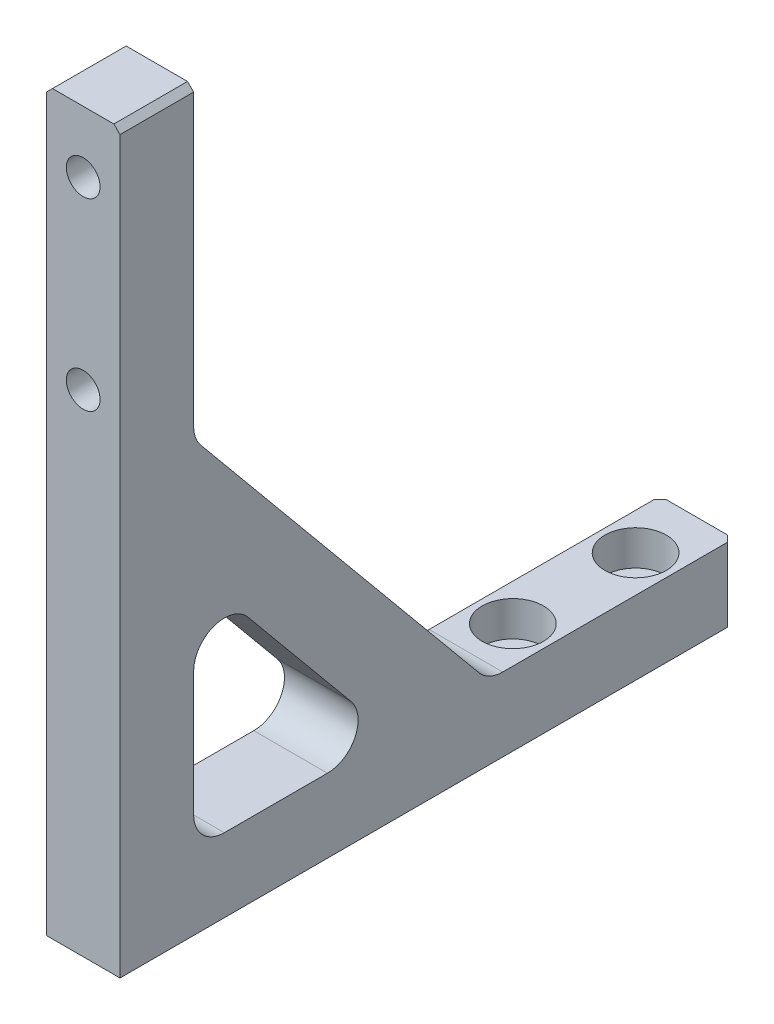
SolidWorks part; units mm, degrees
material "AL6061"
ref_plane "Front Plane" through (0, 0, 0) normal (0, 0, 1) x (1, 0, 0)
ref_plane "Top Plane" through (0, 0, 0) normal (0, 1, 0) x (1, 0, 0)
ref_plane "Right Plane" through (0, 0, 0) normal (1, 0, 0) x (0, 0, -1)
sketch "Sketch1" plane through (0, 0, 0) normal (1, 0, 0) x (0, 0, -1)
  line L0 (0, 0) -> (0, 120)
  line L1 (0, 120) -> (12, 120)
  line L2 (12, 120) -> (12, 70)
  line L3 (12, 70) -> (60, 12)
  line L4 (60, 12) -> (100, 12)
  line L5 (100, 12) -> (100, 0)
  line L6 (100, 0) -> (0, 0)
  dimension "D1" = 12
  dimension "D2" = 12
  dimension "D3" = 120
  dimension "D4" = 100
  dimension "D5" = 40
  dimension "D6" = 50
extrude "Boss-Extrude1" add sketch "Sketch1" along normal blind 12
sketch "Sketch2" plane through (12, 0, 0) normal (1, 0, 0) x (0, 0, -1)
  line L0 (12, 37.2945) -> (12, 17)
  line L1 (17, 12) -> (33.7954, 12)
  line L2 (37.6474, 20.1878) -> (20.852, 40.4823)
  line L3 (12, 70) -> (12, 120) construction
  line L4 (100, 12) -> (60, 12) construction
  line L6 (60, 12) -> (12, 70) construction
  arc A0 (33.7954, 12) -> (37.6474, 20.1878) centre (33.7954, 17) ccw
  arc A1 (12, 17) -> (17, 12) centre (17, 17) ccw
  arc A2 (12, 37.2945) -> (20.852, 40.4823) centre (17, 37.2945) cw
  dimension "D2" = 5
  dimension "D1" = 12
extrude "Cut-Extrude1" cut sketch "Sketch2" against normal through all
hole_wizard "CBORE for M5 Hexagon socket head cap screws1" positions "Sketch3" profile "Sketch4" counterbore size "M5" standard "GB" end condition through all
sketch "Sketch3" plane through (0, 0, -12) normal (0, 0, -1) x (-1, 0, 0)
  line L0 (-6, 120) -> (-6, 0) construction
  line L1 (-12, 120) -> (0, 120) construction
  line L2 (-12, 0) -> (0, 0) construction
  point P9 (-6, 110)
  point P12 (-6, 80)
  dimension "D1" = 80
  dimension "D2" = 30
sketch "Sketch4" plane through (6, 80, -12) normal (1, 0, 0) x (0, 1, 0)
  line L0 (0, 0) -> (0, 12)
  line L1 (0, 12) -> (2.75, 12)
  line L3 (2.75, 12) -> (2.75, 5.7)
  line L4 (2.75, 5.7) -> (5, 5.7)
  line L5 (5, 5.7) -> (5, 0)
  line L7 (5, 0) -> (0, 0)
  line L11 (0, -6.35) -> (0, 107.95) construction
  dimension "通孔孔直径" = 5.5
  dimension "通孔孔深度" = 12
  dimension "柱形沉头孔直径" = 10
  dimension "柱形沉头孔深度" = 5.7
hole_wizard "CBORE for M5 Hexagon socket head cap screws2" positions "Sketch5" profile "Sketch6" counterbore size "M5" standard "GB" end condition through all
sketch "Sketch5" plane through (0, 12, 0) normal (0, 1, 0) x (1, 0, 0)
  line L0 (6, 100) -> (6, 0) construction
  line L1 (12, 100) -> (0, 100) construction
  line L2 (12, 0) -> (0, 0) construction
  point P9 (6, 90)
  point P11 (6, 70)
  dimension "D1" = 70
  dimension "D2" = 20
sketch "Sketch6" plane through (6, 12, -70) normal (1, 0, 0) x (0, 0, 1)
  line L0 (0, 0) -> (0, 12)
  line L1 (0, 12) -> (2.75, 12)
  line L3 (2.75, 12) -> (2.75, 5.7)
  line L4 (2.75, 5.7) -> (5, 5.7)
  line L5 (5, 5.7) -> (5, 0)
  line L7 (5, 0) -> (0, 0)
  line L11 (0, -6.35) -> (0, 107.95) construction
  dimension "通孔孔直径" = 5.5
  dimension "通孔孔深度" = 12
  dimension "柱形沉头孔直径" = 10
  dimension "柱形沉头孔深度" = 5.7
chamfer "Chamfer1" distance 1 angle 45 4 edges at (12, 120, -6) (0, 120, -6) (12, 6, -100) (0, 6, -100)
fillet "Fillet1" radius 5 2 edges at (6, 12, -60) (6, 70, -12)
